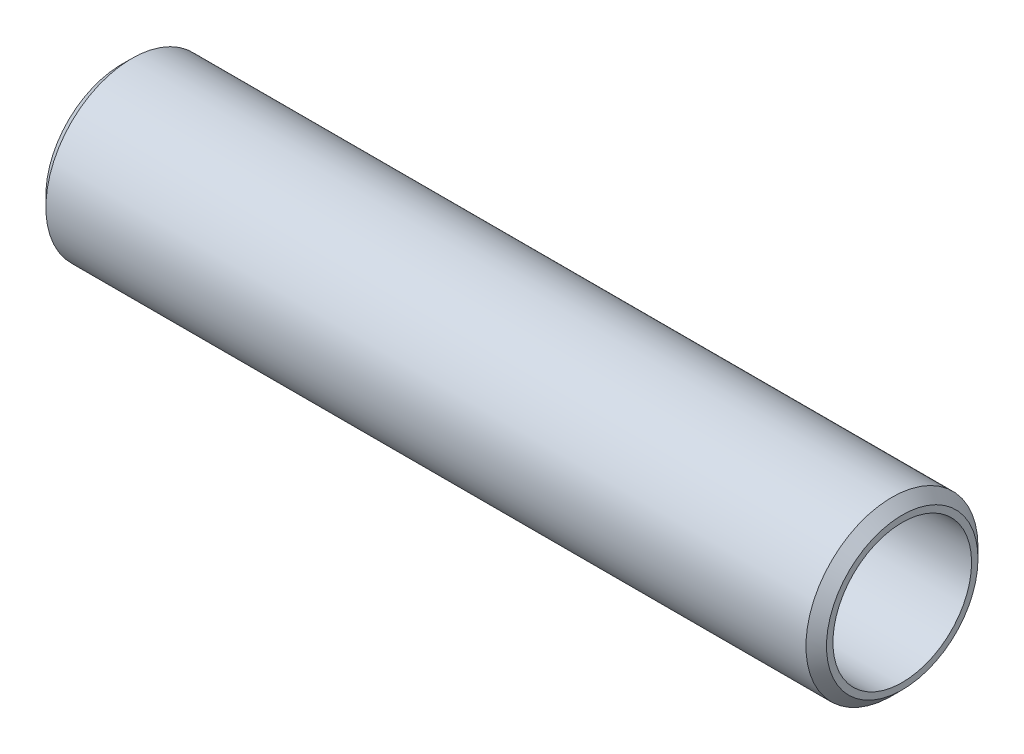
SolidWorks part; units mm, degrees
material "镀锌焊接钢管 Q215A"
ref_plane "前视基准面" through (0, 0, 0) normal (0, 0, 1) x (1, 0, 0)
ref_plane "上视基准面" through (0, 0, 0) normal (0, 1, 0) x (1, 0, 0)
ref_plane "右视基准面" through (0, 0, 0) normal (1, 0, 0) x (0, 0, -1)
sketch "草图1" plane through (0, 0, 0) normal (1, 0, 0) x (0, 0, -1)
  circle A0 centre (0, 0) radius 16.75
  dimension "D1" = 33.5
extrude "拉伸-薄壁1" add sketch "草图1" along normal blind 152 thin thin type one direction reverse wall 3.25
cosmetic thread "装饰螺纹线1" parameters "D1"=20, "D2"=30.291
cosmetic thread "装饰螺纹线2" parameters "D1"=20, "D2"=30.291
chamfer "倒角1" distance 2 angle 45 2 edges at (152, 0, -16.75) (0, 0, -16.75)
